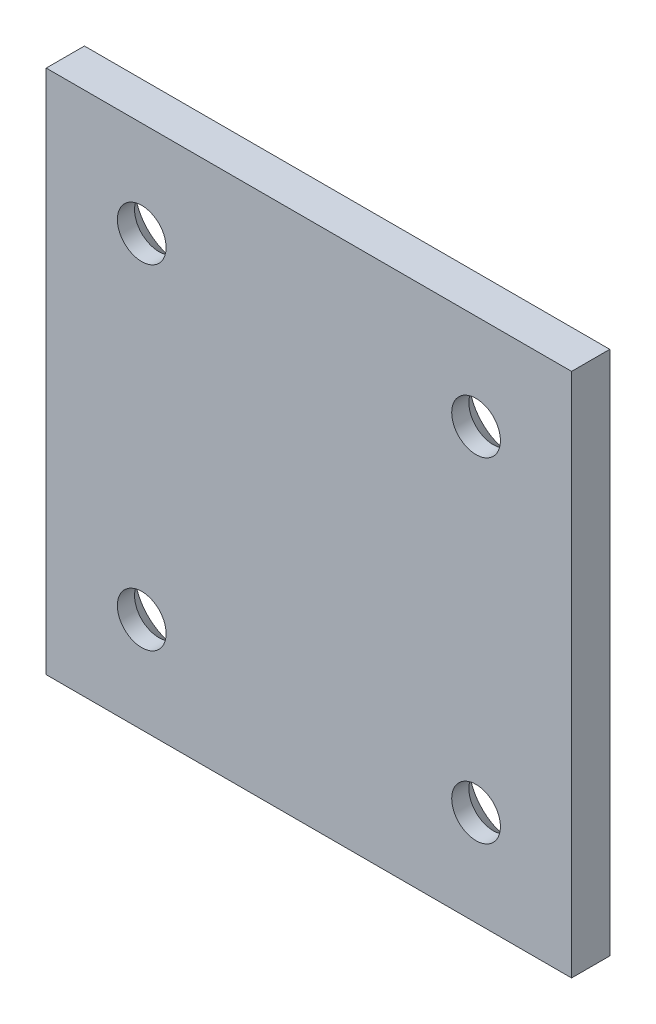
from build123d import *

# Parameters (mm, degrees)
SKETCH1_W                  = 55
SKETCH1_H                  = 55
SKETCH1_W_2                = 35
SKETCH1_H_2                = 35
BOSS_EXTRUDE1_DEPTH        = 4
F_1_0_5_1_DIAMETER_HOLE1_D = 5.1
CHAMFER1_SIZE              = 2.2


with BuildPart() as part:
    # Sketch1 → Boss-Extrude1 (new body)
    # profile 1 of 2: a face of its own
    with BuildSketch(Plane.XY):
        Rectangle(SKETCH1_W, SKETCH1_H)
        Rectangle(SKETCH1_W_2, SKETCH1_H_2, mode=Mode.SUBTRACT)
    # profile 2 of 2: a face of its own
    with BuildSketch(Plane.XY):
        Rectangle(SKETCH1_W_2, SKETCH1_H_2)
    extrude(amount=BOSS_EXTRUDE1_DEPTH)

    # Ø1.0 (5.1) Diameter Hole1 (through all)
    with Locations(Plane(origin=(0, 0, 0), x_dir=(-1, 0, 0), z_dir=(0, 0, -1))):
        with Locations((-17.5, 17.5), (17.5, 17.5), (17.5, -17.5), (-17.5, -17.5)):
            Hole(F_1_0_5_1_DIAMETER_HOLE1_D / 2)

    # Chamfer1
    chamfer1_edges = [part.edges().sort_by_distance(p)[0] for p in [
        (14.95, -17.5, 0),
        (-20.05, -17.5, 0),
        (-20.05, 17.5, 0),
        (14.95, 17.5, 0),
    ]]
    chamfer(chamfer1_edges, length=CHAMFER1_SIZE)


solid = part.part
